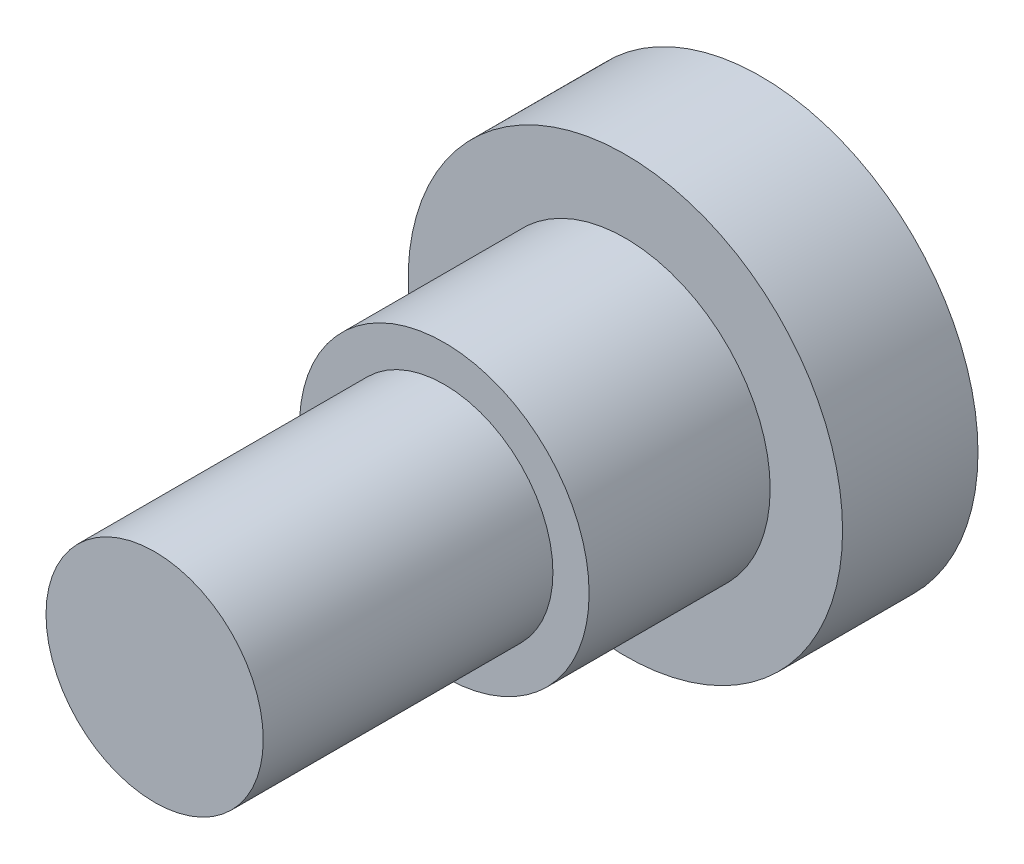
SolidWorks part; units mm, degrees
ref_plane "前视基准面" through (0, 0, 0) normal (0, 0, 1) x (1, 0, 0)
ref_plane "上视基准面" through (0, 0, 0) normal (0, 1, 0) x (1, 0, 0)
ref_plane "右视基准面" through (0, 0, 0) normal (1, 0, 0) x (0, 0, -1)
sketch "草图1" plane through (0, 0, 0) normal (0, 0, 1) x (1, 0, 0)
  circle A0 centre (0, 0) radius 6
  dimension "D1" = 12
extrude "凸台-拉伸1" add sketch "草图1" along normal blind 3.74
sketch "草图2" plane through (0, 0, 3.74) normal (0, 0, 1) x (1, 0, 0)
  circle A0 centre (0, 0) radius 4
  dimension "D1" = 8
extrude "凸台-拉伸2" add sketch "草图2" along normal blind 5
sketch "草图3" plane through (0, 0, 8.74) normal (0, 0, 1) x (1, 0, 0)
  circle A0 centre (0, 0) radius 3
  dimension "D1" = 6
extrude "凸台-拉伸3" add sketch "草图3" along normal blind 8
move or copy body "实体-移动/复制1" [suppressed] bodies to move or copy 103
